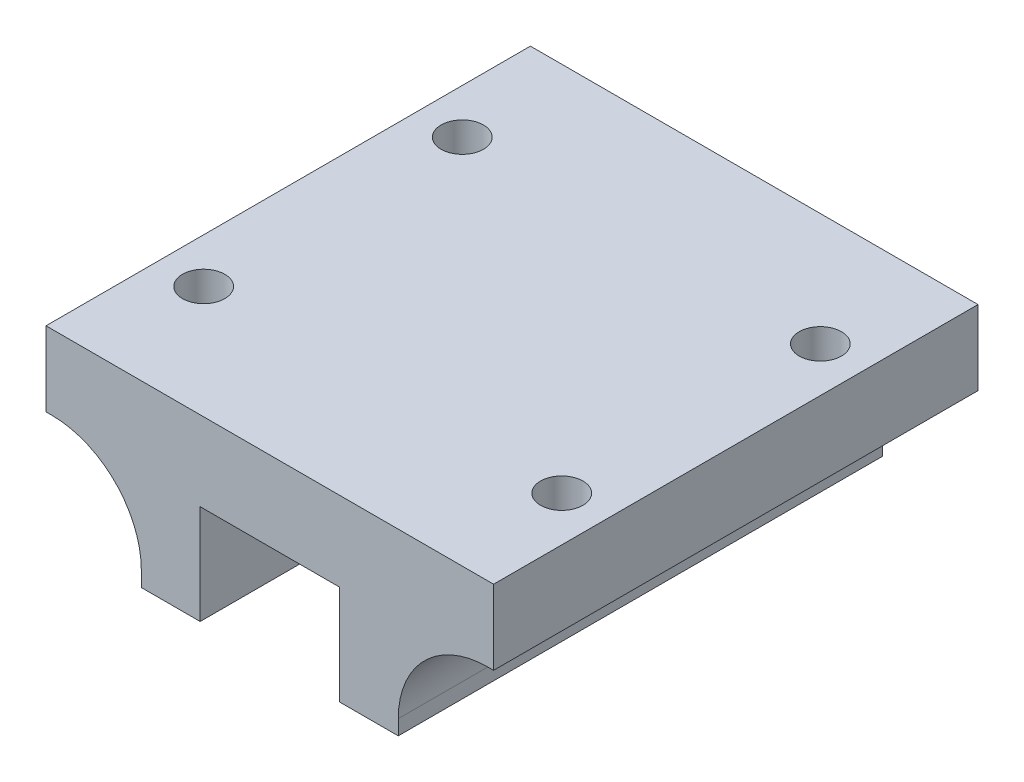
SolidWorks part; units mm, degrees
ref_plane "Front Plane" through (0, 0, 0) normal (0, 0, 1) x (1, 0, 0)
ref_plane "Top Plane" through (0, 0, 0) normal (0, 1, 0) x (1, 0, 0)
ref_plane "Right Plane" through (0, 0, 0) normal (1, 0, 0) x (0, 0, -1)
sketch "Sketch1" plane through (0, 0, 0) normal (0, 0, 1) x (1, 0, 0)
  line L0 (-25.8304, -36) -> (-25.8304, -33)
  line L1 (-45, -15) -> (-45, 0)
  line L2 (-45, 0) -> (45, 0)
  line L3 (45, 0) -> (45, -15)
  line L4 (25.8304, -33) -> (25.8304, -36)
  line L5 (25.8304, -36) -> (14, -36)
  line L6 (0, 0) -> (0, -35) construction
  line L7 (-45, -15) -> (-43.8304, -15)
  line L8 (45, -15) -> (43.8304, -15)
  line L9 (-14, -36) -> (-14, -16)
  line L10 (-14, -16) -> (14, -16)
  line L11 (14, -16) -> (14, -36)
  line L12 (-14, -36) -> (-25.8304, -36)
  arc A0 (-43.8304, -15) -> (-25.8304, -33) centre (-43.8304, -33) cw
  arc A1 (43.8304, -15) -> (25.8304, -33) centre (43.8304, -33) ccw
  dimension "D1" = 28
  dimension "D2" = 90
  dimension "D3" = 36
  dimension "D4" = 20
  dimension "D5" = 15
  dimension "D6" = 3
  dimension "D7" = 11.8304
extrude "Boss-Extrude1" add sketch "Sketch1" along normal mid plane 97.4
hole_wizard "M10 Tapped Hole1" positions "Sketch3" profile "Sketch2" tap size "M10" standard "GB"
sketch "Sketch3" plane through (0, 0, 0) normal (0, 1, 0) x (-1, 0, 0)
  line L0 (0, -48.7) -> (0, 48.7) construction
  line L1 (-45, -48.7) -> (45, -48.7) construction
  line L2 (-45, 48.7) -> (45, 48.7) construction
  line L4 (45, 0) -> (-45, 0) construction
  line L5 (45, 48.7) -> (45, -48.7) construction
  line L6 (-45, 48.7) -> (-45, -48.7) construction
  point P0 (-36, 26)
  point P1 (36, 26)
  point P3 (-36, -26)
  point P5 (36, -26)
  dimension "D1" = 72
  dimension "D2" = 52
sketch "Sketch2" plane through (36, 0, 26) normal (1, 0, 0) x (0, 0, 1)
  line L0 (0, 0) -> (0, 27.0537)
  line L1 (0, 27.0537) -> (4.25, 24.5)
  line L2 (4.25, 24.5) -> (4.25, 0)
  line L5 (4.25, 0) -> (0, 0)
  line L10 (0, 27.0537) -> (-4.25, 24.5) construction
  line L11 (0, -6.35) -> (0, 107.95) construction
  dimension "螺纹孔钻头直径" = 8.5
  dimension "螺纹孔钻头深度" = 24.5
  dimension "导头角度" = 118
cosmetic thread "Cosmetic Thread1" parameters "D1"=20, "D2"=10
cosmetic thread "Cosmetic Thread2" parameters "D1"=20, "D2"=10
cosmetic thread "Cosmetic Thread3" parameters "D1"=20, "D2"=10
cosmetic thread "Cosmetic Thread4" parameters "D1"=20, "D2"=10
